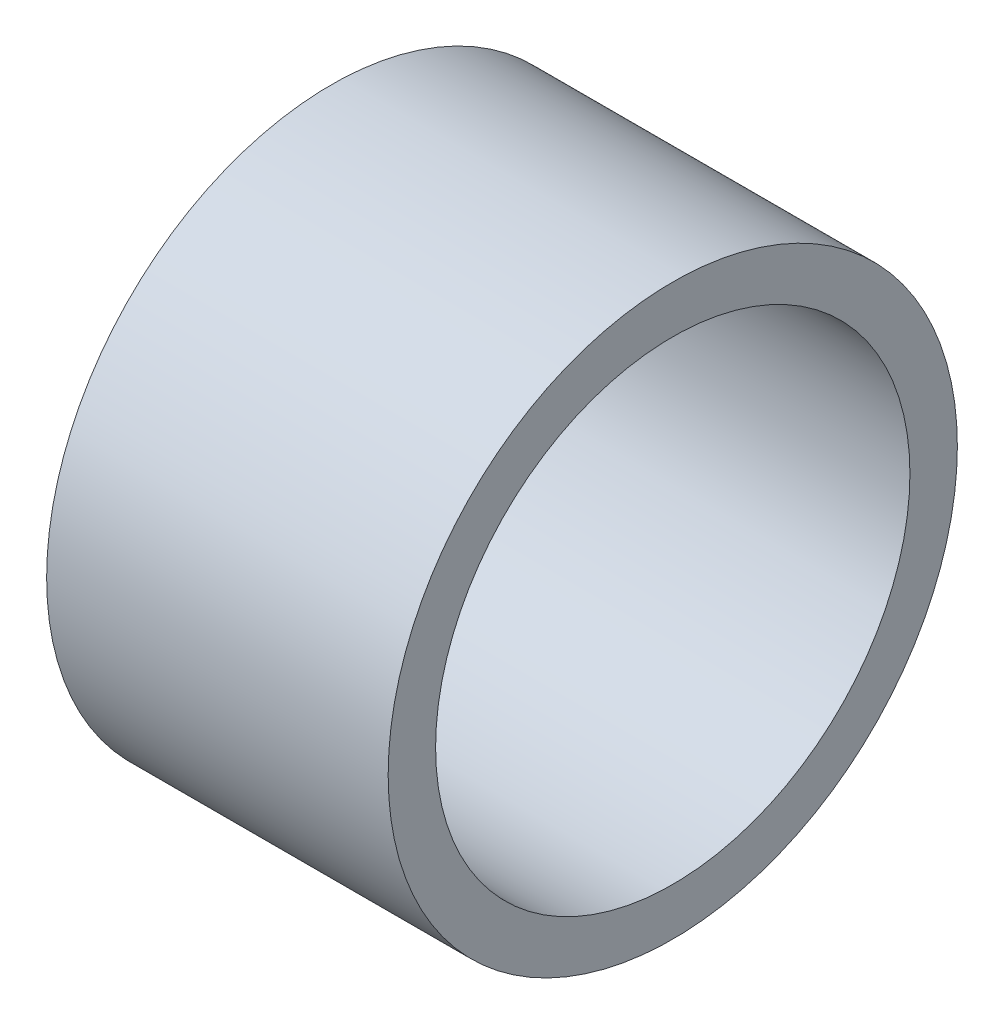
from build123d import *

# Parameters (mm, degrees)
SKETCH1_W = 9
SKETCH1_H = 1.25


with BuildPart() as part:
    # Sketch1 → Revolve1 (revolve)
    with BuildSketch(Plane.XY, mode=Mode.PRIVATE) as revolve1_sk:
        with Locations((4.5, 6.875)):
            Rectangle(SKETCH1_W, SKETCH1_H)
    revolve(revolve1_sk.sketch.rotate(Axis((0, 0, 0), (1, 0, 0)), 90), axis=Axis((0, 0, 0), (1, 0, 0)))


solid = part.part
